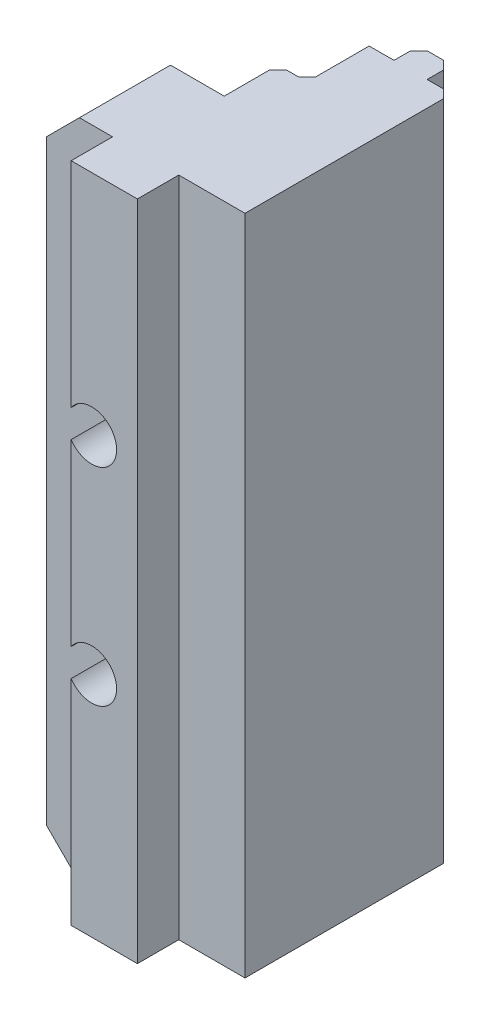
SolidWorks part; units mm, degrees
ref_plane "Front Plane" through (0, 0, 0) normal (0, 0, 1) x (1, 0, 0)
ref_plane "Top Plane" through (0, 0, 0) normal (0, 1, 0) x (1, 0, 0)
ref_plane "Right Plane" through (0, 0, 0) normal (1, 0, 0) x (0, 0, -1)
sketch "Sketch1" plane through (0, 0, 0) normal (0, 1, 0) x (1, 0, 0)
  line L0 (0, 25) -> (0, 0)
  line L1 (0, 0) -> (-24, 0)
  line L2 (-24, 0) -> (-24, 7.0647)
  line L3 (-24, 7.0647) -> (-20.7212, 11)
  line L4 (-20.7212, 11) -> (-13.5115, 11)
  line L5 (-13.5115, 11) -> (-13.5115, 17.5)
  line L6 (-13.5115, 17.5) -> (-10, 17.5)
  line L7 (-10, 17.5) -> (-10, 25)
  line L8 (-10, 25) -> (-7, 25)
  line L9 (-7, 25) -> (-7, 28)
  line L10 (-7, 28) -> (-3, 28)
  line L11 (-3, 28) -> (-3, 25)
  line L12 (-3, 25) -> (0, 25)
  dimension "D1" = 24
  dimension "D2" = 28
  dimension "D3" = 11
  dimension "D4" = 3
  dimension "D5" = 3
  dimension "D6" = 3
  dimension "D7" = 3
  dimension "D8" = 6.5
  dimension "D9" = 4
extrude "Boss-Extrude1" add sketch "Sketch1" along normal blind 80
chamfer "Chamfer1" distance 1 angle 45 5 edges at (-13.5115, 40, -17.5) (0, 40, -25) (-10, 40, -17.5) (-3, 40, -28) (-7, 40, -28)
chamfer "Chamfer2" distance 4 angle 45 2 edges at (-24, 80, -3.5324) (-24, 0, -3.5324)
sketch "Sketch2" plane through (0, 80, 0) normal (0, 1, 0) x (1, 0, 0)
  line L0 (-20, 0) -> (0, 0) construction
  line L1 (-16, 0) -> (-8, 0)
  line L2 (-16, 0) -> (-16, -5)
  line L3 (-16, -5) -> (-8, -5)
  line L4 (-8, 0) -> (-8, -5)
  line L5 (0, 0) -> (0, 24) construction
  dimension "D1" = 8
  dimension "D2" = 5
  dimension "D3" = 8
extrude "Boss-Extrude2" add sketch "Sketch2" against normal blind 80
sketch "Sketch3" plane through (0, 0, -11) normal (0, 0, -1) x (-1, 0, 0)
  line L0 (13.5115, 80) -> (13.5115, 0) construction
  line L1 (13.5115, 40) -> (24, 40) construction
  line L2 (24, 76) -> (24, 4) construction
  line L3 (13.5115, 80) -> (20, 80) construction
  circle A0 centre (13.5115, 52.5) radius 4
  circle A1 centre (13.5115, 27.5) radius 4
  dimension "D1" = 8
  dimension "D2" = 27.5
extrude "Cut-Extrude1" cut sketch "Sketch3" against normal mid plane 15
sketch "Sketch4" plane through (0, 0, -11) normal (0, 0, -1) x (-1, 0, 0)
  line L0 (13.5115, 40) -> (24, 40) construction
  line L1 (13.5115, 48.5) -> (13.5115, 31.5) construction
  line L2 (24, 76) -> (24, 4) construction
  circle A0 centre (13.5115, 52.5) radius 3
  circle A1 centre (13.5115, 27.5) radius 3
  dimension "D1" = 6
extrude "Cut-Extrude2" cut sketch "Sketch4" against normal through all both and the other way through all
sketch "Sketch5" plane through (0, 0, 0) normal (0, 0, 1) x (1, 0, 0)
  line L0 (-24, 76) -> (-24, 4) construction
  line L1 (-24, 40) -> (0, 40) construction
  line L2 (0, 80) -> (0, 0) construction
  line L3 (-16, 0) -> (-16, 25.8244) construction
  circle A0 centre (-19, 40) radius 1.5
  dimension "D1" = 3
  dimension "D2" = 3
extrude "Cut-Extrude3" cut sketch "Sketch5" against normal blind 3 and the other way through all
